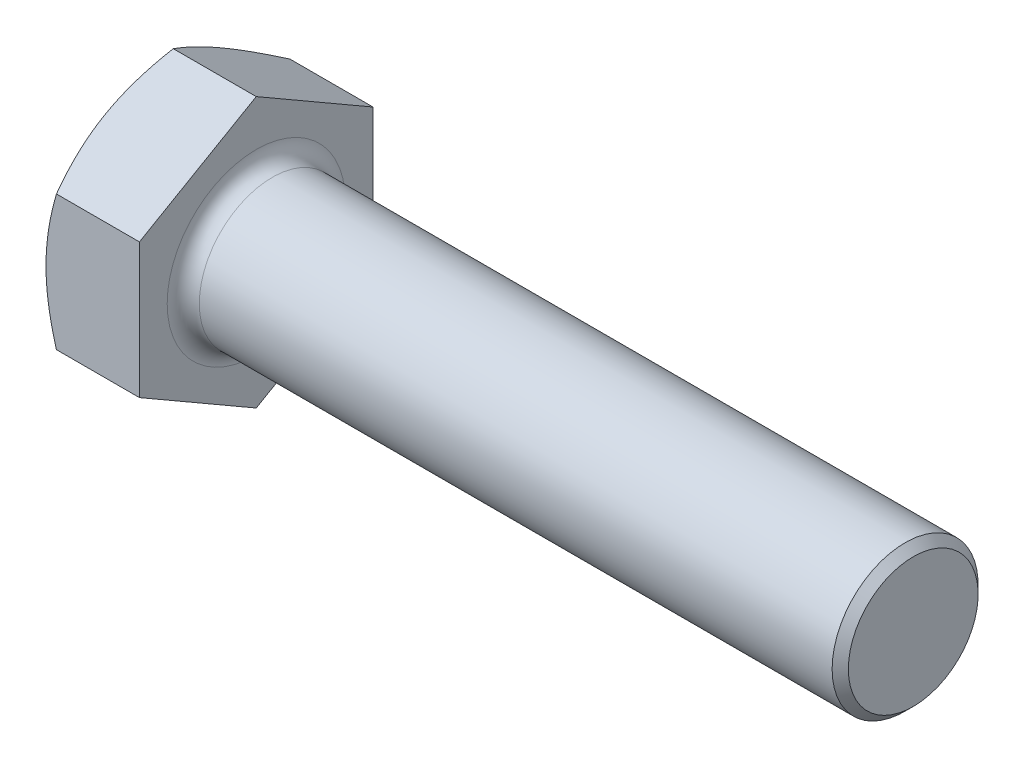
from build123d import *

# Parameters (mm, degrees)
BOSS_EXTRUDE1_DEPTH = 6.4
SKETCH4_R           = 17.59
SKETCH4_R_2         = 8
CUT_EXTRUDE1_DEPTH  = 0.8
CUT_EXTRUDE1_DRAFT  = -60
CHAMFER2_SIZE       = 0.555555556


with BuildPart() as part:
    # Sketch3 → Boss-Extrude1 (new body)
    with BuildSketch(Plane(origin=(0, 0, 0), x_dir=(0, 0, -1), z_dir=(1, 0, 0))):
        Polygon((8, 4.618802154), (0, 9.237604307), (-8, 4.618802154), (-8, -4.618802154), (0, -9.237604307), (8, -4.618802154), align=None)
    extrude(amount=BOSS_EXTRUDE1_DEPTH)


with BuildPart() as cut_extrude1_tool:
    # Sketch4 → Cut-Extrude1 (with draft: the straight prism first)
    with BuildSketch(Plane.ZY):
        Circle(SKETCH4_R)
        Circle(SKETCH4_R_2, mode=Mode.SUBTRACT)
    extrude(amount=-CUT_EXTRUDE1_DEPTH)
    # Cut-Extrude1: the draft: its side faces are tilted about the plane it starts from
    cut_extrude1_sides = [cut_extrude1_tool.faces().sort_by_distance(p)[0] for p in [
        (0.4, 0, -17.59),
        (0.4, 0, -8),
    ]]
    draft(cut_extrude1_sides, Plane.ZY, CUT_EXTRUDE1_DRAFT)


with BuildPart() as part_1:
    add(part.part)

    # Cut-Extrude1: cut by cut_extrude1_tool
    add(cut_extrude1_tool.part, mode=Mode.SUBTRACT)

    # Sketch5 → Revolve1 (revolve)
    with BuildSketch(Plane.XY, mode=Mode.PRIVATE) as revolve1_sk:
        with BuildLine():
            Line((7.5, 5), (51.4, 5))
            Line((51.4, 5), (51.4, 0))
            Line((51.4, 0), (6.4, 0))
            Line((6.4, 0), (6.4, 6.1))
            ThreePointArc((6.4, 6.1), (6.722182541, 5.322182541), (7.5, 5))
        make_face()
    revolve(revolve1_sk.sketch.rotate(Axis((6.4, 0, 0), (1, 0, 0)), 90), axis=Axis((6.4, 0, 0), (1, 0, 0)))

    # Chamfer2
    chamfer2_edges = [part_1.edges().sort_by_distance(p)[0] for p in [
        (51.4, 0, -5),
    ]]
    chamfer(chamfer2_edges, length=CHAMFER2_SIZE)


solid = part_1.part
